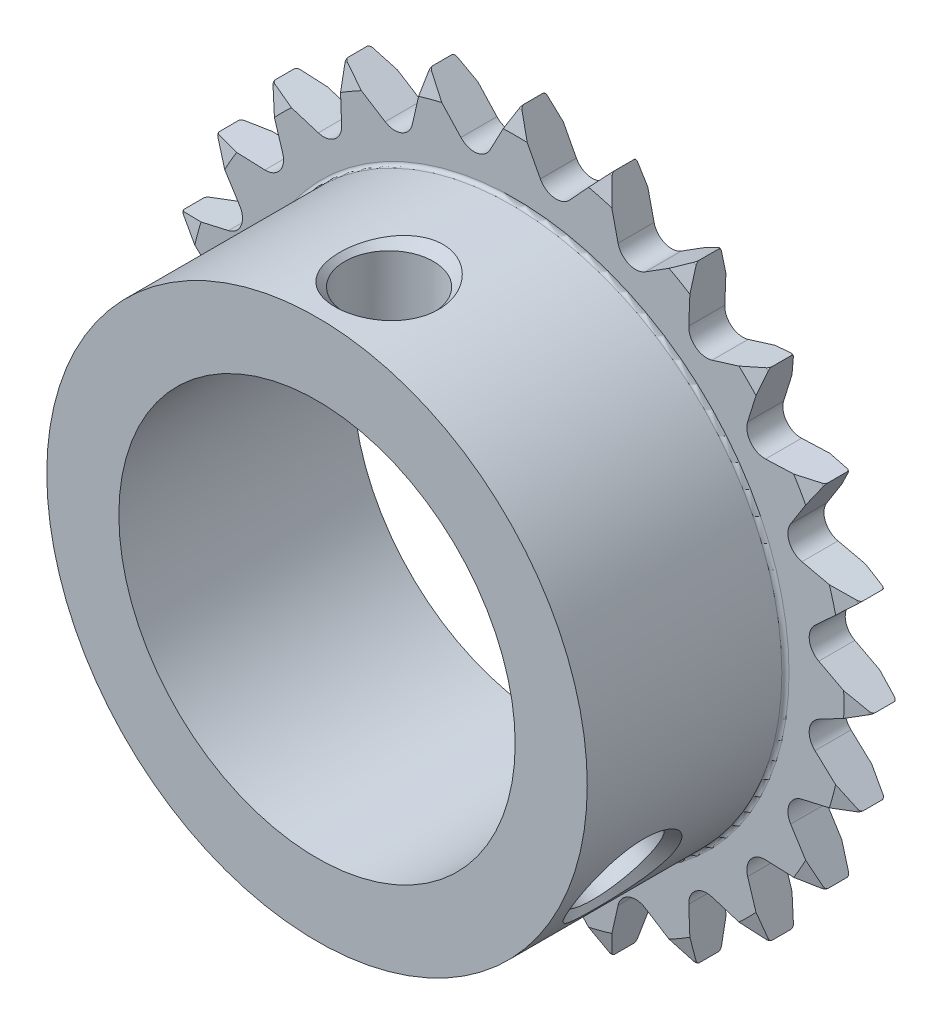
from build123d import *

# Parameters (mm, degrees)
SKETCH_2_W               = 302.005499825
SKETCH_2_H               = 246.129864536
CUT_EXTRUDE_1_DEPTH      = 2
CUT_EXTRUDE_2_DEPTH      = 32.882597256
CUT_EXTRUDE_2_DEPTH_BACK = 32.882597256
SKETCH_5_W               = 33.679256415
SKETCH_5_H               = 3
SKETCH_6_R               = 11
CUT_EXTRUDE_3_DEPTH      = 31.487702609


with BuildPart() as part:
    # 草图1 → 旋转1 (revolve)
    with BuildSketch(Plane(origin=(0, 0, 0), x_dir=(0, 0, -1), z_dir=(1, 0, 0)), mode=Mode.PRIVATE) as revolve_1_sk:
        with BuildLine():
            Line((-16, 7.7), (-15.8, 7.5))
            Line((-15.8, 7.5), (-0.2, 7.5))
            Line((-0.2, 7.5), (0, 7.7))
            Line((0, 7.7), (0, 18.245))
            Line((0, 18.245), (-0.296556469, 19.351763809))
            ThreePointArc((-0.296556469, 19.351763809), (-0.367989348, 19.458670668), (-0.489741634, 19.5))
            Line((-0.489741634, 19.5), (-1.510258366, 19.5))
            ThreePointArc((-1.510258366, 19.5), (-1.632010652, 19.458670668), (-1.703443531, 19.351763809))
            Line((-1.703443531, 19.351763809), (-2, 18.245))
            Line((-2, 18.245), (-2, 15.2))
            ThreePointArc((-2, 15.2), (-2.058578644, 15.058578644), (-2.2, 15))
            Line((-2.2, 15), (-15.8, 15))
            Line((-15.8, 15), (-16, 14.8))
            Line((-16, 14.8), (-16, 7.7))
        make_face()
    revolve(revolve_1_sk.sketch.rotate(Axis((0, 0, 0), (0, 0, 1)), 270), axis=Axis((0, 0, 0), (0, 0, 1)))

    # 草图2 → 切除-拉伸1 (cut)
    with BuildSketch(Plane.XY):
        with Locations((0.692673165, 3.694256879)):
            Rectangle(SKETCH_2_W, SKETCH_2_H)
        with BuildLine():
            Line((-19.5, 0), (-16.851187604, -1.395063166))
            ThreePointArc((-16.851187604, -1.395063166), (-16.325738013, -2.149324184), (-16.638066227, -3.013880743))
            Line((-16.638066227, -3.013880743), (-18.835553613, -5.046971379))
            Line((-18.835553613, -5.046971379), (-15.915928394, -5.708935826))
            ThreePointArc((-15.915928394, -5.708935826), (-15.213165947, -6.301499662), (-15.291088132, -7.217433661))
            Line((-15.291088132, -7.217433661), (-16.887495374, -9.75))
            Line((-16.887495374, -9.75), (-13.896024966, -9.633753943))
            ThreePointArc((-13.896024966, -9.633753943), (-13.063841762, -10.024238351), (-12.902047651, -10.929130401))
            Line((-12.902047651, -10.929130401), (-13.788582233, -13.788582233))
            Line((-13.788582233, -13.788582233), (-10.929130401, -12.902047651))
            ThreePointArc((-10.929130401, -12.902047651), (-10.024238351, -13.063841762), (-9.633753943, -13.896024966))
            Line((-9.633753943, -13.896024966), (-9.75, -16.887495374))
            Line((-9.75, -16.887495374), (-7.217433661, -15.291088132))
            ThreePointArc((-7.217433661, -15.291088132), (-6.301499662, -15.213165947), (-5.708935826, -15.915928394))
            Line((-5.708935826, -15.915928394), (-5.046971379, -18.835553613))
            Line((-5.046971379, -18.835553613), (-3.013880743, -16.638066227))
            ThreePointArc((-3.013880743, -16.638066227), (-2.149324184, -16.325738013), (-1.395063166, -16.851187604))
            Line((-1.395063166, -16.851187604), (0, -19.5))
            Line((0, -19.5), (1.395063166, -16.851187604))
            ThreePointArc((1.395063166, -16.851187604), (2.149324184, -16.325738013), (3.013880743, -16.638066227))
            Line((3.013880743, -16.638066227), (5.046971379, -18.835553613))
            Line((5.046971379, -18.835553613), (5.708935826, -15.915928394))
            ThreePointArc((5.708935826, -15.915928394), (6.301499662, -15.213165947), (7.217433661, -15.291088132))
            Line((7.217433661, -15.291088132), (9.75, -16.887495374))
            Line((9.75, -16.887495374), (9.633753943, -13.896024966))
            ThreePointArc((9.633753943, -13.896024966), (10.024238351, -13.063841762), (10.929130401, -12.902047651))
            Line((10.929130401, -12.902047651), (13.788582233, -13.788582233))
            Line((13.788582233, -13.788582233), (12.902047651, -10.929130401))
            ThreePointArc((12.902047651, -10.929130401), (13.063841762, -10.024238351), (13.896024966, -9.633753943))
            Line((13.896024966, -9.633753943), (16.887495374, -9.75))
            Line((16.887495374, -9.75), (15.291088132, -7.217433661))
            ThreePointArc((15.291088132, -7.217433661), (15.213165947, -6.301499662), (15.915928394, -5.708935826))
            Line((15.915928394, -5.708935826), (18.835553613, -5.046971379))
            Line((18.835553613, -5.046971379), (16.638066227, -3.013880743))
            ThreePointArc((16.638066227, -3.013880743), (16.325738013, -2.149324184), (16.851187604, -1.395063166))
            Line((16.851187604, -1.395063166), (19.5, 0))
            Line((19.5, 0), (16.851187604, 1.395063166))
            ThreePointArc((16.851187604, 1.395063166), (16.325738013, 2.149324184), (16.638066227, 3.013880743))
            Line((16.638066227, 3.013880743), (18.835553613, 5.046971379))
            Line((18.835553613, 5.046971379), (15.915928394, 5.708935826))
            ThreePointArc((15.915928394, 5.708935826), (15.213165947, 6.301499662), (15.291088132, 7.217433661))
            Line((15.291088132, 7.217433661), (16.887495374, 9.75))
            Line((16.887495374, 9.75), (13.896024966, 9.633753943))
            ThreePointArc((13.896024966, 9.633753943), (13.063841762, 10.024238351), (12.902047651, 10.929130401))
            Line((12.902047651, 10.929130401), (13.788582233, 13.788582233))
            Line((13.788582233, 13.788582233), (10.929130401, 12.902047651))
            ThreePointArc((10.929130401, 12.902047651), (10.024238351, 13.063841762), (9.633753943, 13.896024966))
            Line((9.633753943, 13.896024966), (9.75, 16.887495374))
            Line((9.75, 16.887495374), (7.217433661, 15.291088132))
            ThreePointArc((7.217433661, 15.291088132), (6.301499662, 15.213165947), (5.708935826, 15.915928394))
            Line((5.708935826, 15.915928394), (5.046971379, 18.835553613))
            Line((5.046971379, 18.835553613), (3.013880743, 16.638066227))
            ThreePointArc((3.013880743, 16.638066227), (2.149324184, 16.325738013), (1.395063166, 16.851187604))
            Line((1.395063166, 16.851187604), (0, 19.5))
            Line((0, 19.5), (-1.395063166, 16.851187604))
            ThreePointArc((-1.395063166, 16.851187604), (-2.149324184, 16.325738013), (-3.013880743, 16.638066227))
            Line((-3.013880743, 16.638066227), (-5.046971379, 18.835553613))
            Line((-5.046971379, 18.835553613), (-5.708935826, 15.915928394))
            ThreePointArc((-5.708935826, 15.915928394), (-6.301499662, 15.213165947), (-7.217433661, 15.291088132))
            Line((-7.217433661, 15.291088132), (-9.75, 16.887495374))
            Line((-9.75, 16.887495374), (-9.633753943, 13.896024966))
            ThreePointArc((-9.633753943, 13.896024966), (-10.024238351, 13.063841762), (-10.929130401, 12.902047651))
            Line((-10.929130401, 12.902047651), (-13.788582233, 13.788582233))
            Line((-13.788582233, 13.788582233), (-12.902047651, 10.929130401))
            ThreePointArc((-12.902047651, 10.929130401), (-13.063841762, 10.024238351), (-13.896024966, 9.633753943))
            Line((-13.896024966, 9.633753943), (-16.887495374, 9.75))
            Line((-16.887495374, 9.75), (-15.291088132, 7.217433661))
            ThreePointArc((-15.291088132, 7.217433661), (-15.213165947, 6.301499662), (-15.915928394, 5.708935826))
            Line((-15.915928394, 5.708935826), (-18.835553613, 5.046971379))
            Line((-18.835553613, 5.046971379), (-16.638066227, 3.013880743))
            ThreePointArc((-16.638066227, 3.013880743), (-16.325738013, 2.149324184), (-16.851187604, 1.395063166))
            Line((-16.851187604, 1.395063166), (-19.5, 0))
        make_face(mode=Mode.SUBTRACT)
    extrude(amount=CUT_EXTRUDE_1_DEPTH, mode=Mode.SUBTRACT)

    # 草图3 → 切除-旋转1 (revolve, cut)
    with BuildSketch(Plane.XY.offset(9), mode=Mode.PRIVATE) as cut_revolve_1_sk:
        Polygon((0, 2.3), (-3, 2.3), (-3, 9.8), (-2.4585, 10.3415), (-2.4585, 14.4585), (-3, 15), (-3, 22.5), (0, 22.5), align=None)
    revolve(cut_revolve_1_sk.sketch.rotate(Axis((0, 15, 9), (0, -1, 0)), 180), axis=Axis((0, 15, 9), (0, -1, 0)), mode=Mode.SUBTRACT)

    # 草图4 → 切除-旋转2 (revolve, cut)
    with BuildSketch(Plane.XY.offset(9), mode=Mode.PRIVATE) as cut_revolve_2_sk:
        Polygon((0, 0), (1.5, 2.598076211), (7.995190528, -1.151923789), (8.193393285, -1.891626545), (13.750678301, -5.100126545), (14.490381057, -4.901923789), (20.985571585, -8.651923789), (19.485571585, -11.25), align=None)
    revolve(cut_revolve_2_sk.sketch.rotate(Axis((12.990381057, -7.5, 9), (-0.8660254037844384, 0.5000000000000007, 0)), 180), axis=Axis((12.990381057, -7.5, 9), (-0.8660254037844384, 0.5000000000000007, 0)), mode=Mode.SUBTRACT)

    # 草图5 → 切除-拉伸2 (cut, two sides: drawn at the far end of the back side and taken through both)
    with BuildSketch(Plane(origin=(0, 0, 0), x_dir=(1, 0, 0), z_dir=(0, 1, 0)).offset(-CUT_EXTRUDE_2_DEPTH_BACK)):
        with Locations((1.072716701, -14.5)):
            Rectangle(SKETCH_5_W, SKETCH_5_H)
    extrude(amount=CUT_EXTRUDE_2_DEPTH + CUT_EXTRUDE_2_DEPTH_BACK, mode=Mode.SUBTRACT)

    # 草图6 → 切除-拉伸3 (cut, through all)
    with BuildSketch(Plane(origin=(0, 0, 0), x_dir=(-1, 0, 0), z_dir=(0, 0, -1))):
        Circle(SKETCH_6_R)
    extrude(amount=-CUT_EXTRUDE_3_DEPTH, mode=Mode.SUBTRACT)


solid = part.part
